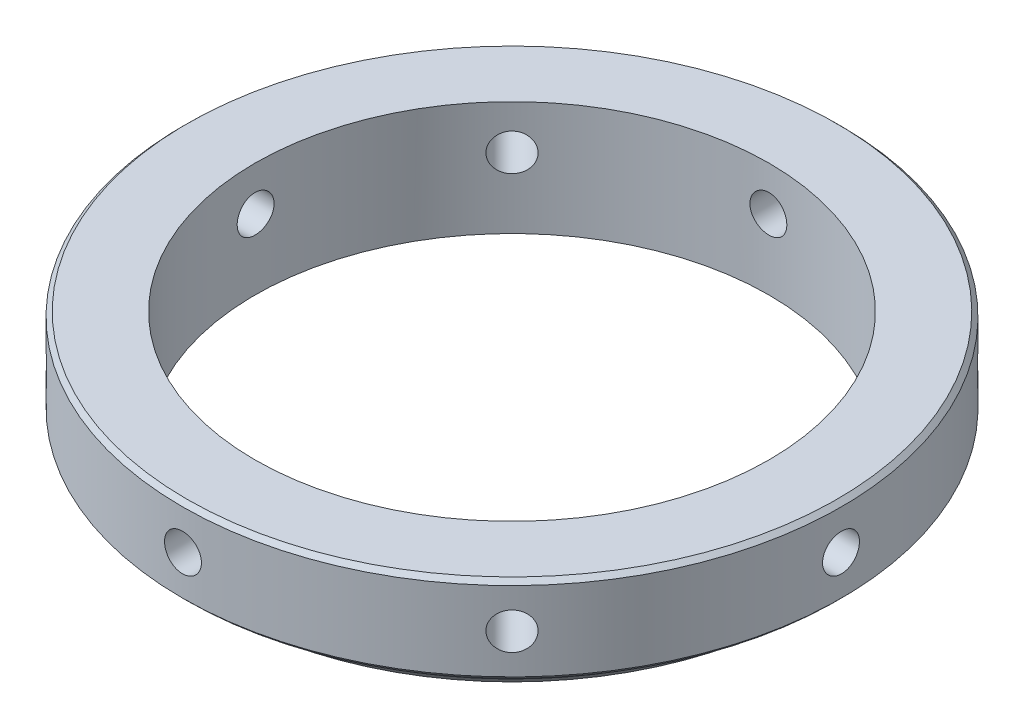
from build123d import *

# Parameters (mm, degrees)
SKETCH_1_R               = 37.5
SKETCH_1_R_2             = 29.25
EXTRUDE_1_DEPTH          = 5
PATTERN_CIRCULAR_1_COUNT = 8
CHAMFER_1_SIZE           = 0.5
EXTRUDE_START            = 3
SKETCH_6_R               = 34.25
SKETCH_6_R_2             = 29.25
EXTRUDE_2_DEPTH          = 3
CHAMFER_2_SIZE           = 1


with BuildPart() as part:
    # 草图1 → 凸台-拉伸1 (new, symmetric)
    with BuildSketch(Plane(origin=(0, 0, 0), x_dir=(1, 0, 0), z_dir=(0, 1, 0))):
        with Locations(Location((0, 0, 0), (0, 0, 270))):
            Circle(SKETCH_1_R)
        with Locations(Location((0, 0, 0), (0, 0, 270))):
            Circle(SKETCH_1_R_2, mode=Mode.SUBTRACT)
    extrude(amount=EXTRUDE_1_DEPTH, both=True)

    # 草图2 → Ø4.2 (4.2) 直径孔1 (revolve, cut)
    with BuildSketch(Plane(origin=(0, 0, 40), x_dir=(0, -1, 0), z_dir=(1, 0, 0))):
        Polygon((0, 0), (0, 16.2618073), (2.1, 15), (2.1, 0), align=None)
    hole_wizard_4_2_4_2_1 = revolve(axis=Axis((0, 0, 46.35), (0, 0, -1)), mode=Mode.SUBTRACT)

    # 阵列(圆周)1: Ø4.2 (4.2) 直径孔1 ×8 about axis
    pattern_circular_1_axis = Axis((0, 5, 0), (0, -1, 0))
    for i in range(1, PATTERN_CIRCULAR_1_COUNT):
        add(hole_wizard_4_2_4_2_1.rotate(pattern_circular_1_axis, i * 360 / PATTERN_CIRCULAR_1_COUNT), mode=Mode.SUBTRACT)

    # 倒角1
    chamfer_1_edges = [part.edges().sort_by_distance(p)[0] for p in [
        (0, -5, -37.5),
        (0, 5, -37.5),
    ]]
    chamfer(chamfer_1_edges, length=CHAMFER_1_SIZE)

    # 草图6 → 凸台-拉伸2 (add)
    with BuildSketch(Plane.XZ.offset(5).offset(EXTRUDE_START)):
        with Locations(Location((0, 0, 0), (0, 0, 90))):
            Circle(SKETCH_6_R)
        with Locations(Location((0, 0, 0), (0, 0, 270))):
            Circle(SKETCH_6_R_2, mode=Mode.SUBTRACT)
    extrude(amount=-EXTRUDE_2_DEPTH)

    # 倒角2
    chamfer_2_edges = [part.edges().sort_by_distance(p)[0] for p in [
        (0, -8, -34.25),
    ]]
    chamfer(chamfer_2_edges, length=CHAMFER_2_SIZE)


solid = part.part
